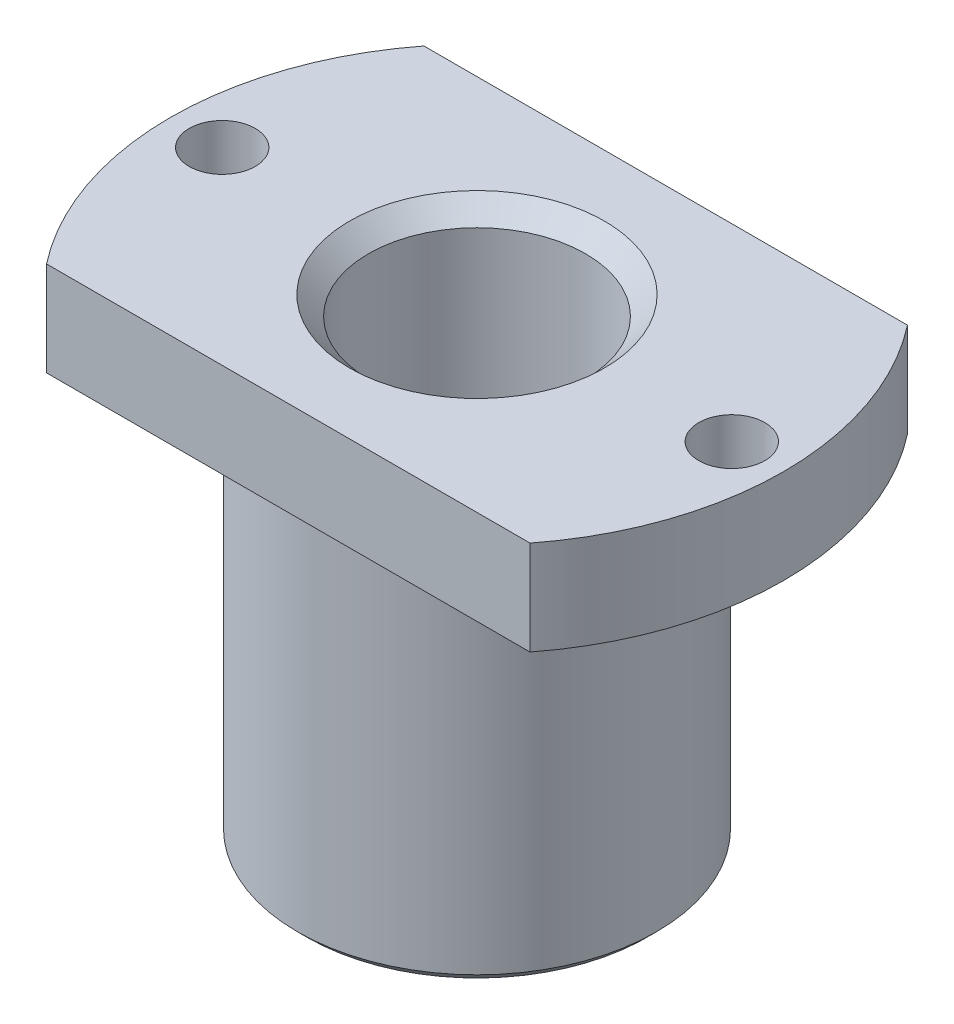
from build123d import *

# Parameters (mm, degrees)
SKETCH1_R           = 19
BOSS_EXTRUDE1_DEPTH = 50
SKETCH2_R           = 32.5
BOSS_EXTRUDE2_DEPTH = 10
CUT_EXTRUDE1_REACH  = 69.915
SKETCH3_R           = 11.5
SKETCH4_R           = 3.5
CUT_EXTRUDE2_DEPTH  = 61.930288035
CIRPATTERN1_COUNT   = 4
CHAMFER1_SIZE       = 1
CHAMFER2_SIZE       = 2
CUT_EXTRUDE3_REACH  = 69.915


with BuildPart() as part:
    # Sketch1 → Boss-Extrude1 (new body)
    with BuildSketch(Plane(origin=(0, 0, 0), x_dir=(1, 0, 0), z_dir=(0, 1, 0))):
        with Locations(Location((0, 0, 0), (0, 0, 270))):
            Circle(SKETCH1_R)
    extrude(amount=BOSS_EXTRUDE1_DEPTH)

    # Sketch2 → Boss-Extrude2 (add)
    with BuildSketch(Plane(origin=(0, 50, 0), x_dir=(1, 0, 0), z_dir=(0, 1, 0))):
        with Locations(Location((0, 0, 0), (0, 0, 270))):
            Circle(SKETCH2_R)
    extrude(amount=-BOSS_EXTRUDE2_DEPTH)

    # Sketch3 → Cut-Extrude1 (cut, up to next)
    with BuildSketch(Plane.XZ, mode=Mode.PRIVATE) as cut_extrude1_sk1:
        with Locations(Location((0, 0, 0), (0, 0, 270))):
            Circle(SKETCH3_R)
    cut_extrude1_tool1 = extrude(cut_extrude1_sk1.sketch, amount=-CUT_EXTRUDE1_REACH, mode=Mode.PRIVATE) & part.part
    cut_extrude1 = cut_extrude1_tool1.solids().sort_by_distance((0, 0, 0))[0]
    add(cut_extrude1, mode=Mode.SUBTRACT)

    # Sketch4 → Cut-Extrude2 (cut, through all)
    with BuildSketch(Plane.XZ.offset(-40)):
        with Locations(Location((-27, 0, 0), (0, 0, 270))):
            Circle(SKETCH4_R)
    cut_extrude2 = extrude(amount=-CUT_EXTRUDE2_DEPTH, mode=Mode.SUBTRACT)

    # CirPattern1: Cut-Extrude1, Cut-Extrude2 ×4 about axis
    cirpattern1_axis = Axis((0, 0, 0), (0, 1, 0))
    add([cut_extrude1.rotate(cirpattern1_axis, i * 360 / CIRPATTERN1_COUNT) for i in range(1, CIRPATTERN1_COUNT)], mode=Mode.SUBTRACT)
    add([cut_extrude2.rotate(cirpattern1_axis, i * 360 / CIRPATTERN1_COUNT) for i in range(1, CIRPATTERN1_COUNT)], mode=Mode.SUBTRACT)

    # Chamfer1
    chamfer1_edges = [part.edges().sort_by_distance(p)[0] for p in [
        (0, 0, -19),
    ]]
    chamfer(chamfer1_edges, length=CHAMFER1_SIZE)

    # Chamfer2
    chamfer2_edges = [part.edges().sort_by_distance(p)[0] for p in [
        (0, 50, 11.5),
        (0, 0, 11.5),
    ]]
    chamfer(chamfer2_edges, length=CHAMFER2_SIZE)

    # Sketch5 → Cut-Extrude3 (cut, up to next)
    with BuildSketch(Plane(origin=(0, 50, 0), x_dir=(1, 0, 0), z_dir=(0, 1, 0)), mode=Mode.PRIVATE) as cut_extrude3_sk1:
        with BuildLine():
            Line((-25.617376915, -20), (25.617376915, -20))
            ThreePointArc((25.617376915, -20), (0, -32.5), (-25.617376915, -20))
        make_face()
    cut_extrude3_tool1 = extrude(cut_extrude3_sk1.sketch, amount=-CUT_EXTRUDE3_REACH, mode=Mode.PRIVATE) & part.part
    # Sketch5 → Cut-Extrude3 (cut, up to next)
    with BuildSketch(Plane(origin=(0, 50, 0), x_dir=(1, 0, 0), z_dir=(0, 1, 0)), mode=Mode.PRIVATE) as cut_extrude3_sk2:
        with BuildLine():
            Line((-25.617376915, 20), (25.617376915, 20))
            ThreePointArc((25.617376915, 20), (0, 32.5), (-25.617376915, 20))
        make_face()
    cut_extrude3_tool2 = extrude(cut_extrude3_sk2.sketch, amount=-CUT_EXTRUDE3_REACH, mode=Mode.PRIVATE) & part.part
    add(cut_extrude3_tool1.solids().sort_by_distance((0, 50, 25.09283))[0], mode=Mode.SUBTRACT)
    add(cut_extrude3_tool2.solids().sort_by_distance((0, 50, -25.09283))[0], mode=Mode.SUBTRACT)


solid = part.part
